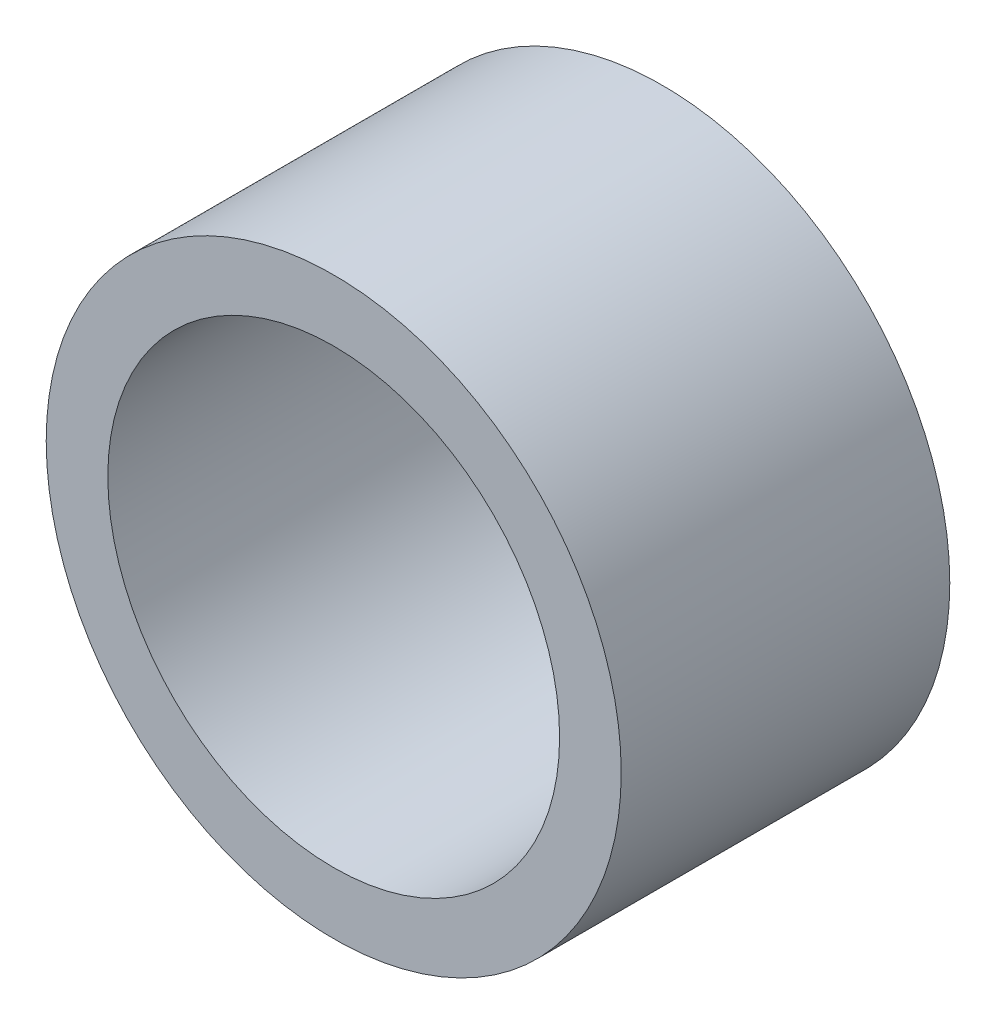
from build123d import *

# Parameters (mm, degrees)
SKETCH_1_R      = 35
SKETCH_1_R_2    = 27.5
EXTRUDE_1_DEPTH = 40


with BuildPart() as part:
    # 草图1 → 凸台-拉伸1 (new body)
    with BuildSketch(Plane.XY):
        Circle(SKETCH_1_R)
        Circle(SKETCH_1_R_2, mode=Mode.SUBTRACT)
    extrude(amount=EXTRUDE_1_DEPTH)


solid = part.part
